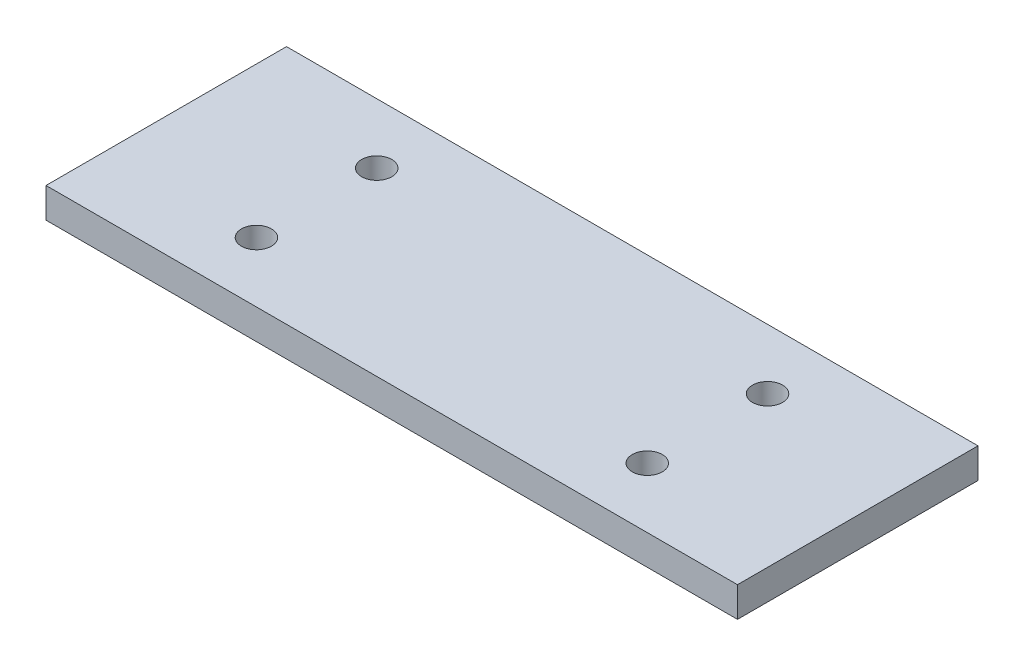
SolidWorks part; units mm, degrees
ref_plane "Front Plane" through (0, 0, 0) normal (0, 0, 1) x (1, 0, 0)
ref_plane "Top Plane" through (0, 0, 0) normal (0, 1, 0) x (1, 0, 0)
ref_plane "Right Plane" through (0, 0, 0) normal (1, 0, 0) x (0, 0, -1)
sketch "Sketch1" plane through (0, 0, 0) normal (0, 0, 1) x (1, 0, 0)
  line L1 (-57.5, 2.5) -> (57.5, 2.5)
  line L2 (-57.5, 2.5) -> (-57.5, -2.5)
  line L3 (-57.5, -2.5) -> (57.5, -2.5)
  line L4 (57.5, 2.5) -> (57.5, -2.5)
  line L5 (-57.5, 2.5) -> (57.5, -2.5) construction
  line L6 (-57.5, -2.5) -> (57.5, 2.5) construction
  point P0 (0, 0)
  dimension "D1" = 5
  dimension "D2" = 115
extrude "Boss-Extrude1" add sketch "Sketch1" against normal blind 40
sketch "Sketch2" plane through (0, 2.5, 0) normal (0, 1, 0) x (1, 0, 0)
  line L0 (-57.5, 40) -> (-57.5, 0) construction
  line L1 (57.5, 40) -> (-57.5, 40) construction
  line L2 (57.5, 0) -> (-57.5, 0) construction
  circle A0 centre (-32.5, 30) radius 2.5
  circle A1 centre (32.5, 30) radius 2.5
  circle A2 centre (-32.5, 10) radius 2.5
  circle A3 centre (32.5, 10) radius 2.5
  dimension "D1" = 5
  dimension "D2" = 5
  dimension "D3" = 5
  dimension "D4" = 5
  dimension "D5" = 25
  dimension "D6" = 25
  dimension "D7" = 65
  dimension "D8" = 65
  dimension "D9" = 10
  dimension "D10" = 10
  dimension "D11" = 10
extrude "Cut-Extrude1" cut sketch "Sketch2" against normal blind 40
